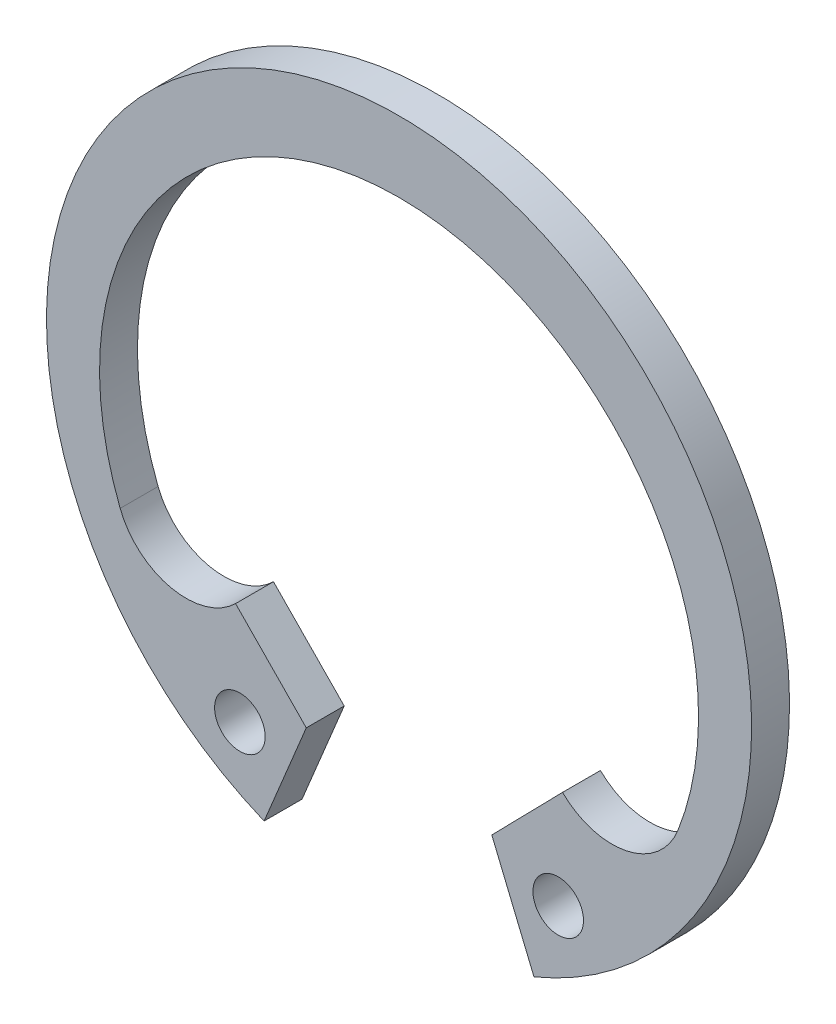
SolidWorks part; units mm, degrees
ref_plane "前视" through (0, 0, 0) normal (0, 0, 1) x (1, 0, 0)
ref_plane "上视" through (0, 0, 0) normal (0, 1, 0) x (1, 0, 0)
ref_plane "右视" through (0, 0, 0) normal (1, 0, 0) x (0, 0, -1)
sketch "草图1" plane through (0, 0, 0) normal (0, 0, 1) x (1, 0, 0)
  line L0 (0, -11.8766) -> (0, 11.8063) construction
  line L1 (0, 0) -> (-4.6199, -11.1535) construction
  line L2 (-6.468, -6.0015) -> (-3.6699, -8.86)
  line L3 (-3.6699, -8.86) -> (-5.3384, -12.8881)
  line L4 (3.6699, -8.86) -> (5.3384, -12.8881)
  line L5 (6.468, -6.0015) -> (3.6699, -8.86)
  arc A0 (5.3384, -12.8881) -> (-5.3384, -12.8881) centre (0, 0) ccw
  arc A1 (11.0338, -5.0218) -> (-11.0338, -5.0218) centre (0, -0.7) ccw
  circle A2 centre (-6.2981, -9.9787) radius 1
  arc A3 (-11.0338, -5.0218) -> (-6.468, -6.0015) centre (-8.4267, -4.0006) ccw
  circle A4 centre (6.2981, -9.9787) radius 1
  arc A5 (11.0338, -5.0218) -> (6.468, -6.0015) centre (8.4267, -4.0006) cw
sketch "尺寸草图" plane through (0, 0, 0) normal (0, 0, 1) x (1, 0, 0)
  line L0 (-13.95, 0) -> (13.95, 0) construction
  line L1 (0, 0) -> (29.4981, -33.9833) construction
  circle A2 centre (0, 0) radius 13.95
  point P9 (9.75, 0)
  point P10 (10.45, 0)
  point P11 (-9, 0)
  point P12 (-5.8, 0)
  point P13 (4.36, 0)
  point P14 (-9.8, 0)
  point P15 (-13.8, 0)
  point P16 (-11.8, 0)
  point P18 (0.7866, -0.9062)
extrude "基体-拉伸" add sketch "草图1" along normal blind 1.5
equation "\"D1@草图1\" = \"DD@尺寸草图\""
equation "\"D2@草图1\" = \"d@尺寸草图\""
equation "\"D5@草图1\" = \"R2@尺寸草图\""
equation "\"D9@草图1\" = \"R@尺寸草图\""
equation "\"D7@草图1\" = \"B@尺寸草图\""
equation "\"D10@草图1\" = \"B1@尺寸草图\""
equation "\"D4@草图1\" = \"d1@尺寸草图\""
equation "\"D6@草图1\" = \"a@尺寸草图\""
equation "\"D8@草图1\" = \"aa@尺寸草图\"/2"
equation "\"D3@草图1\" = \"c@尺寸草图\""
equation "\"D1@基体-拉伸\"=\"s@尺寸草图\"/2"
equation "\"D2@基体-拉伸\" = \"D1@基体-拉伸\""
